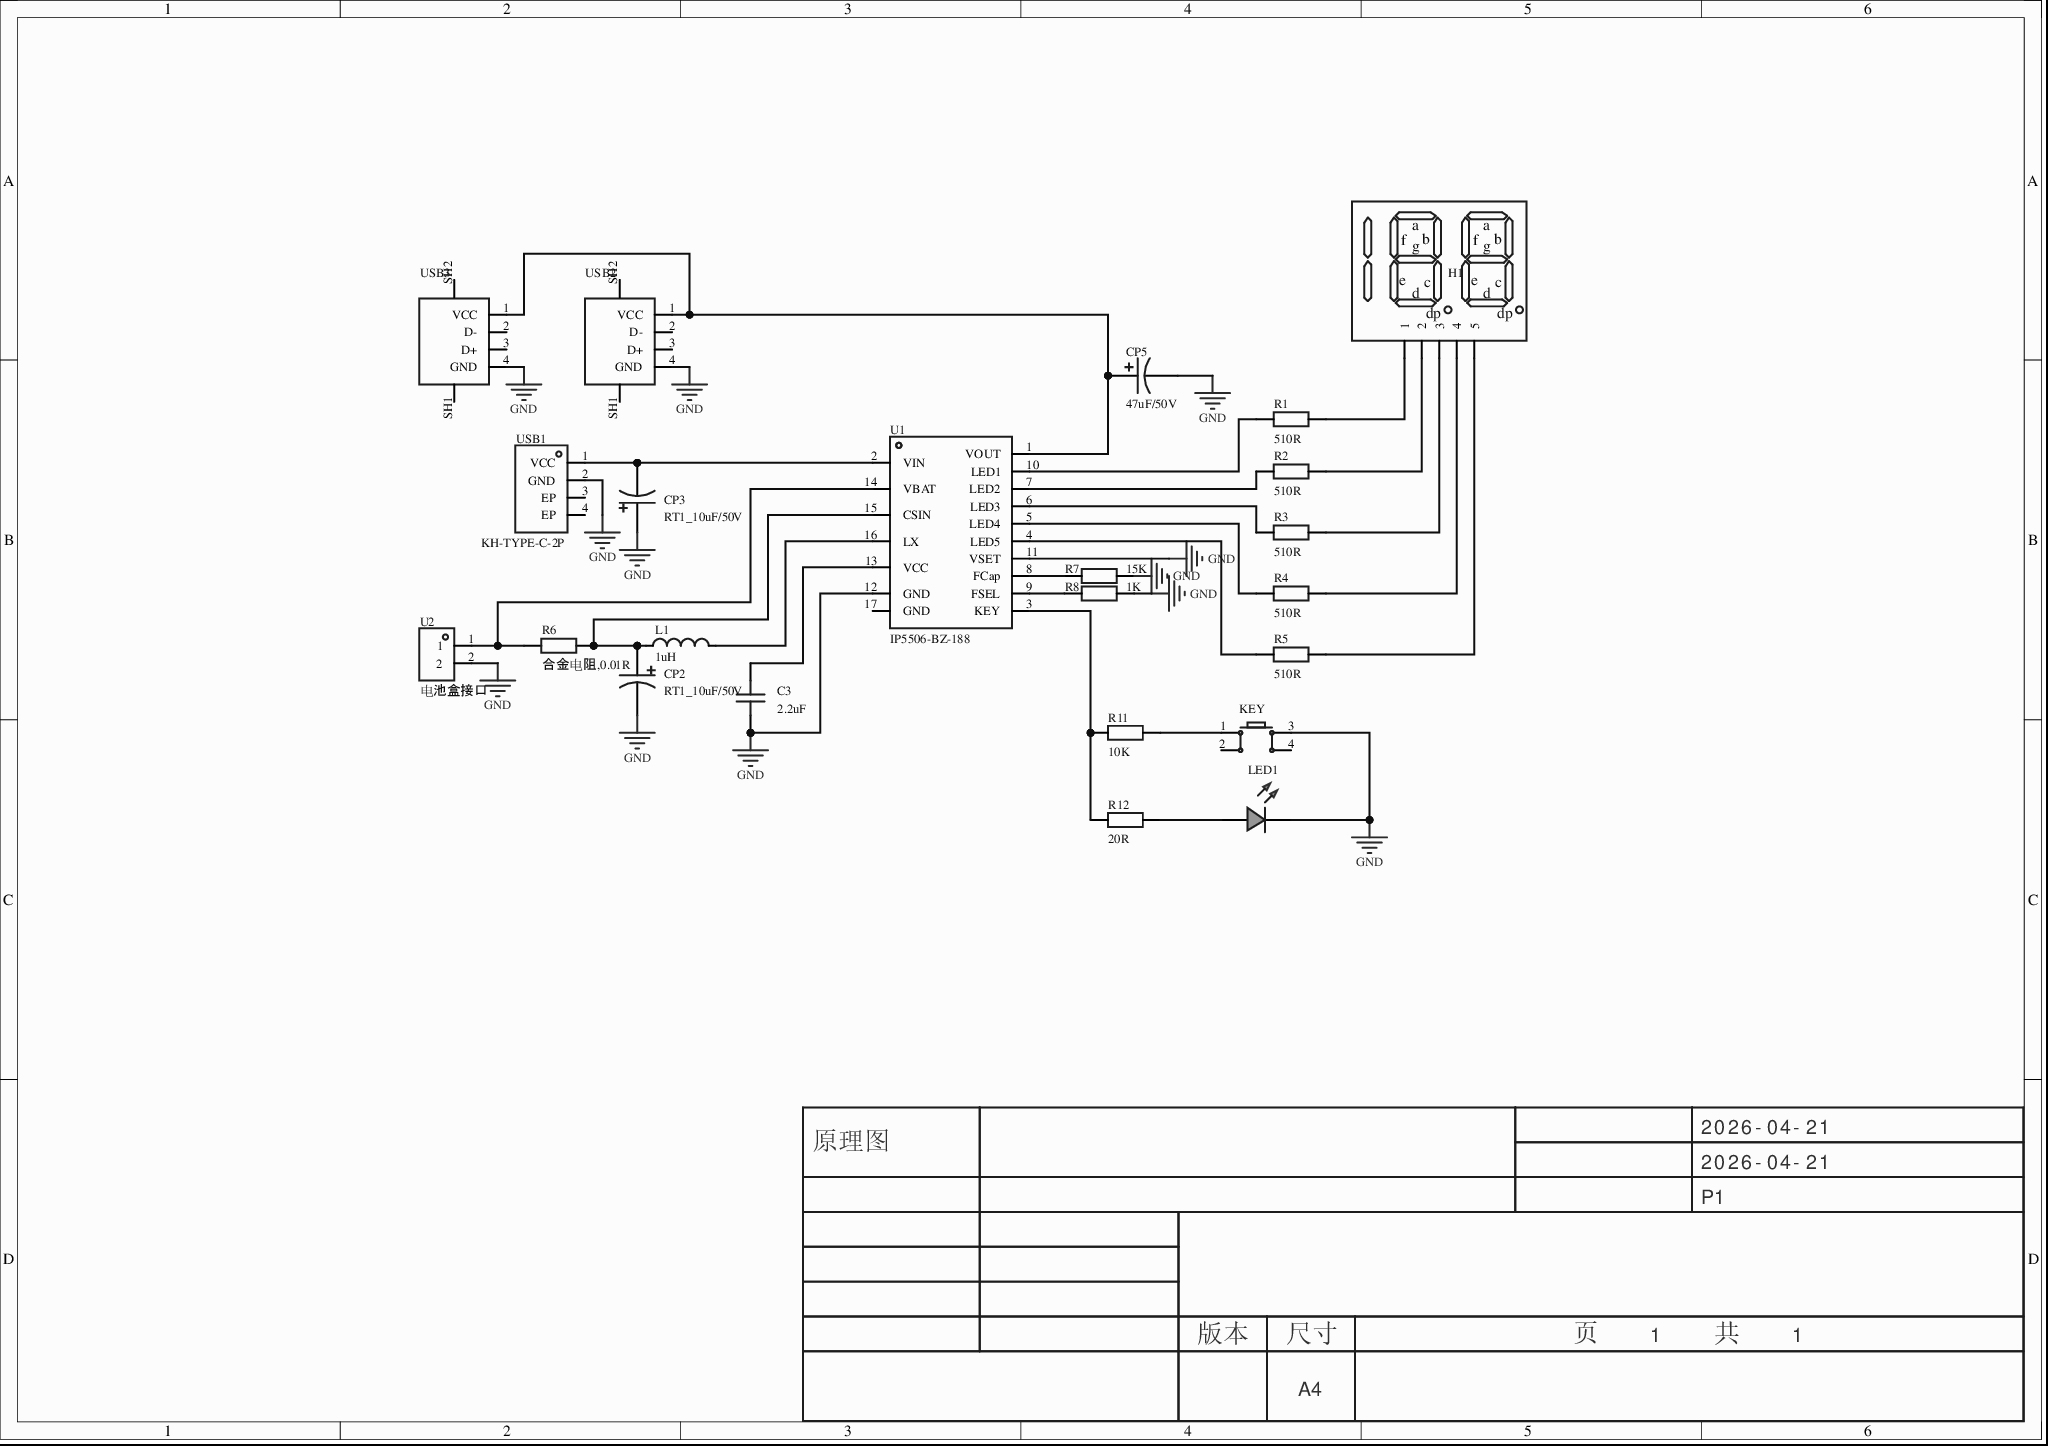
[diagram p0: MISC51911-3.schdoc]
# Altium project MISC51911-2.PrjPcb
1 sheet, 23 parts. Net scope: global (net labels, ports and power ports of the same name join across sheets).
Board file: MISC51911.pcbdoc

## Sheet MISC51911-3.schdoc
size 297 x 209 mm; Version: V1.0; @Project Name: MISC51911; @Update Date: 2026-04-21; @Create Date: 2026-04-21; @Board Name: MISC51911; @Create Time: 23:40:13; @Page Count: 1; @Page No: 1; @Schematic Name: MISC51911; @Update Time: 23:40:13; Size: A4

### Parts
C3  2.2uF  [C0805]
CP2  RT1_10uF/50V  [CAP-TH_BD5.0-P2.00-D0.8-FD]
CP3  RT1_10uF/50V  [CAP-TH_BD5.0-P2.00-D0.8-FD]
CP5  47uF/50V  [CAP-SMD_BD6.3-L6.6-W6.6-LS7.0-FD]
H1  (no value)  [HDR-TH_5P-P2.54-V-F]
KEY  (no value)  [SW-TH_4P-L6.0-W6.0-P4.50-LS6.5]
L1  1uH  [IND-SMD_L7.0-W6.6]
LED1  (no value)  [LED-TH_5mm]
R1  510R  [R0805]
R2  510R  [R0805]
R3  510R  [R0805]
R4  510R  [R0805]
R5  510R  [R0805]
R6  合金电阻,0.01R  [R1206]
R7  15K  [R0805]
R8  1K  [R0805]
R11  10K  [R0805]
R12  20R  [R0805]
U1  IP5506-BZ-188  [ESOP-16_L9.9-W3.9-P1.27-LS6.0-BL-EP]
U2  电池盒接口  [TH_C9900019910]
USB1  KH-TYPE-C-2P  [USB-SMD_KH-TYPE-C-2P]
USB2  (no value)  [USB_ Type-A]
USB3  (no value)  [USB_ Type-A]

### Nets
GND: C3.1 CP2.2 CP3.1 CP5.2 KEY.3 LED1.2(A) R7.2 R8.2 U1.11(VSET) U1.12(GND) U2.2 USB1.2(GND) USB2.4(GND) USB3.4(GND)
NetC3_2: C3.2 U1.13(VCC)
NetCP2_1: CP2.1 L1.1 R6.2 U1.15(CSIN)
NetCP3_2: CP3.2 U1.2(VIN) USB1.1(VCC)
NetCP5_1: CP5.1 U1.1(VOUT) USB2.1(VCC) USB3.1(VCC)
NetH1_1: H1.1 R1.2
NetH1_2: H1.2 R2.2
NetH1_3: H1.3 R3.2
NetH1_4: H1.4 R4.2
NetH1_5: H1.5 R5.2
NetKEY_1: KEY.1 R11.2
NetL1_2: L1.2 U1.16(LX)
NetLED1_1: LED1.1(C) R12.2
NetR1_1: R1.1 U1.10(LED1)
NetR2_1: R2.1 U1.7(LED2)
NetR3_1: R3.1 U1.6(LED3)
NetR4_1: R4.1 U1.5(LED4)
NetR5_1: R5.1 U1.4(LED5)
NetR6_1: R6.1 U1.14(VBAT) U2.1
NetR7_1: R7.1 U1.8(FCap)
NetR8_1: R8.1 U1.9(FSEL)
NetR11_1: R11.1 R12.1 U1.3(KEY)

Not connected (* = marked no-connect by the designer): KEY 2 4; U1 17(GND); USB1 3(EP) 4(EP); USB2 2(D-) 3(D+) SH1 SH2; USB3 2(D-) 3(D+) SH1 SH2

### Notes on the sheet
- 2026-04-21
- 原理图
- P1
- 版本
- 尺寸
- A4
- 页    1    共    1

### Library data of the parts
C3 = CAP_0805: Symbol: Capacitance; ConvertToPcb: yes; ModelId: 1ba041120af144c991958decab20d2410819f05c4eef4c71ace90d822a990e87; ModelName: C0805_L2.0-W1.3-H1.3; ModelTransform: 78.74,51.181,0,0,0,0,0,0.0005,0; Device: CAP_0805; Value: 2.2uF; AddInBom: yes; Supplier Footprint: 0805; FootprintName: C0805
CP2 CP3 = RT1_10uF/50V: AddInBom: yes; ModelId: edeeed87cbc746108d01291548c386360819f05c4eef4c71ace90d822a990e87; ModelName: CAP-TH_D5.0×H7.0×P2.0; ModelTransform: 197.091,196.7911,0,0,0,0,0,0,-137.795; Symbol: RT1_10UF/50V; Device: RT1_10uF/50V; LCSC Part Name: RT1_10uF/50V; SupplierPart: C9900092014; ManufacturerPart: RT1_10uF/50V; Supplier Footprint: CAP2.0*5*11; JLCPCB Part Class: Extended Part; Supplier: LCSC; ConvertToPcb: yes; FootprintName: CAP-TH_BD5.0-P2.00-D0.8-FD
CP5 = 47uF/50V: AddInBom: yes; ModelId: 4a341388e7b34cb7b0bbc1bc8ba36d450819f05c4eef4c71ace90d822a990e87; ModelName: CAP-SMD_BD6.3-L6.6-W6.6-H7.7; ModelTransform: 275.59,259.842,0,0,0,0,0,0,0; Symbol: 47UF/50V; Device: 47uF/50V; LCSC Part Name: 47uF/50V; SupplierPart: C9900005030; ManufacturerPart: 47uF/50V; Supplier Footprint: CAP-SMD_BD6.3-L6.6-W6.6-LS7.0; JLCPCB Part Class: Extended Part; Supplier: LCSC; ConvertToPcb: yes; FootprintName: CAP-SMD_BD6.3-L6.6-W6.6-LS7.0-FD
H1 = HDR-F_2.54_1x5P: Symbol: Header-Female-2.54_1x5_1; ConvertToPcb: yes; ModelId: f49cb6116a3d45e5a64915bf3e00773f0819f05c4eef4c71ace90d822a990e87; ModelTransform: 519.684,98.464,0,0,0,0,0,0,-124.016; Device: HDR-F_2.54_1x5P; AddInBom: yes; SupplierPart: C50950; Supplier Footprint: 插件; FootprintName: HDR-TH_5P-P2.54-V-F; ModelName: HDR-TH_5P-P2.54-V-F
KEY = Key_TH_6x6x6: 触点电流:50mA;额定电压(DC):12V;绝缘电阻:100MΩ;电路结构:单刀单掷;安装方式:直插;按钮形状:圆形按钮;按钮/盖帽颜色:黑色;作用力:260gf@±30gf;工作温度:-25℃~+70℃;引脚样式:PC引脚;开关长度:6mm;开关宽度:6mm;开关高度:6mm;带支架:否;; Symbol: 轻触按键; AddInBom: yes; ModelId: 20eee248bc684ccd8cbdbb1d0d91ec6f0819f05c4eef4c71ace90d822a990e87; ModelName: SW-TH_4P-L6.0-W6.0-H5.0-LS6.5-P4.50; ModelTransform: 236.22,323.03,0,90,0,0,0,0,-137.795; Device: Key_TH_6x6x6; ConvertToPcb: yes; FootprintName: SW-TH_4P-L6.0-W6.0-P4.50-LS6.5; Supplier Footprint: 插件
L1 = SPM70701R0MESL: 电感值:1uH;精度:±20%;饱和电流(Isat):15A;; AddInBom: yes; ModelId: 6860c29aec394a38a0f014af7f722a420819f05c4eef4c71ace90d822a990e87; ModelName: IND-SMD_L7.0-W6.6-H3.0; ModelTransform: 275.59,259.88137,0,0,0,0,0,0,0; Tolerance: ±20%; Current - Saturation(Isat): 15A; DC Resistance(DCR): 8.5mΩ; Symbol: SPM70701R0MESL; Device: SPM70701R0MESL; LCSC Part Name: 1uH ±20% 15A; SupplierPart: C5332207; ManufacturerPart: SPM70701R0MESL; Supplier Footprint: SMD,6.9x6.6mm; JLCPCB Part Class: Extended Part; Datasheet: https://item.szlcsc.com/datasheet/SPM70701R0MESL/6092943.html; Supplier: LCSC; ConvertToPcb: yes; FootprintName: IND-SMD_L7.0-W6.6; Value: 1uH
LED1 = LED_TH-G_5mm: ConvertToPcb: yes; ModelId: fe7796f666a04da4b4289311169b45200819f05c4eef4c71ace90d822a990e87; ModelName: LED-TH_BD5.8-P2.54-FD_GREEN-1; ModelTransform: 212.58,227.91,537.36,0,0,0,-7.87,0,-196.85; Symbol: LED_TH-G; Device: LED_TH-G_5mm; AddInBom: yes; Supplier Footprint: 插件; FootprintName: LED-TH_5mm
R1-R5 R7 R8 R11 R12 = Res_0805: Symbol: 电阻; ConvertToPcb: yes; ModelId: 37a81e68749a4138bd2dfa6897b24b850819f05c4eef4c71ace90d822a990e87; ModelName: R0805_L2.0-W1.3-H0.6; ModelTransform: 78.74,51.181,0,0,0,0,0,-0.0005,0; Device: Res_0805; AddInBom: yes; Supplier Footprint: 0805; FootprintName: R0805
  R1-R5: Value: 510R
  R7: Value: 15K
  R8: Value: 1K
  R11: Value: 10K
  R12: Value: 20R
R6 = 合金电阻,0.1R,+/-1%,R1206,1W.: AddInBom: yes; ModelId: 89a1f13db2384da588040e0b3c55bf660819f05c4eef4c71ace90d822a990e87; ModelName: R1206_L3.2-W1.6-H0.6; ModelTransform: 125.984,62.992,0,0,0,0,0,0,0; Symbol: 合金电阻,0.1R,+/-1%,R1206,1W.; Device: 合金电阻,0.1R,+/-1%,R1206,1W.; Manufacturer Part: 合金电阻,0.01R; LCSC Part Name: 合金电阻,0.1R,+/-1%,R1206,1W.; SupplierPart: C9900011777; Supplier Footprint: R1206; JLCPCB Part Class: Extended Part; Supplier: LCSC; ConvertToPcb: yes; FootprintName: R1206
U1 = IP5506-BZ-188: Symbol: IP5506-BZ-188_1; AddInBom: yes; ModelId: 7a4e8929b80a410c8bd84dfe389bd4c40819f05c4eef4c71ace90d822a990e87; ModelName: ESOP-16_L10.0-W3.9-H1.7-LS6.0-P1.27; ModelTransform: 240.157,393.701,0,90,0,0,0,0.0055,0; Device: IP5506-BZ-188; LCSC Part Name: IC; SupplierPart: C605441; ManufacturerPart: IP5506-BZ-188; Supplier Footprint: ESOP-16; JLCPCB Part Class: Extended Part; Supplier: LCSC; ConvertToPcb: yes; FootprintName: ESOP-16_L9.9-W3.9-P1.27-LS6.0-BL-EP
U2 = 电池盒接口: AddInBom: yes; Symbol: 电池盒接口; Device: 电池盒接口; LCSC Part Name: 电池盒接口; SupplierPart: C9900019910; ManufacturerPart: 电池盒接口; Supplier Footprint: 2pin-焊盘; JLCPCB Part Class: Extended Part; Supplier: LCSC; ConvertToPcb: yes; FootprintName: TH_C9900019910
USB1 = KH-TYPE-C-2P: 连接器类型:Type-C;协议标准:-;公母:-;安装方式:弯插;触点数量:2P;端口数量:1;额定电流 - 电源:3A;工作温度:-25℃~+85℃;; Manufacturer: kinghelm(金航标); AddInBom: yes; ModelId: 4464b34a7d0f48c2b8c2350e914c93f50819f05c4eef4c71ace90d822a990e87; ModelTransform: 352.362,255.31449,0,0,0,0,0,-49.213,-98.425; Connector Type: Type-C; Number of Contacts: 2P; Number of Ports: 1; Current Rating-Power: 3A; Voltage Rating: 20V; Connect-Disconnect Life: 5千次; Symbol: KH-TYPE-C-2P; Device: KH-TYPE-C-2P; LCSC Part Name: Type-C 弯插; SupplierPart: C2919656; ManufacturerPart: KH-TYPE-C-2P; Supplier Footprint: 插件; JLCPCB Part Class: Extended Part; Datasheet: https://item.szlcsc.com/datasheet/KH-TYPE-C-2P/3222638.html; Supplier: LCSC; ConvertToPcb: yes; FootprintName: USB-SMD_KH-TYPE-C-2P; ModelName: USB-SMD_KH-TYPE-C-2P; Protocol Standard: -; Gender: -; Mounting Type: 弯插; Length: 6.43mm; Operating Temperature: -25℃~+85℃
USB2 USB3 = USB_ Type-A: AddInBom: yes; ModelId: 0a0bfc60af8549fa93b7465d8aaf02b10819f05c4eef4c71ace90d822a990e87; ModelName: USB-A-TH__USB-AF-90; ModelTransform: 612.05,551.18,446.85,0,0,0,0,-15.75,-157.48; Symbol: USB_Type-A; Device: USB_ Type-A; ConvertToPcb: yes; FootprintName: USB_ Type-A; Supplier Footprint: 插件